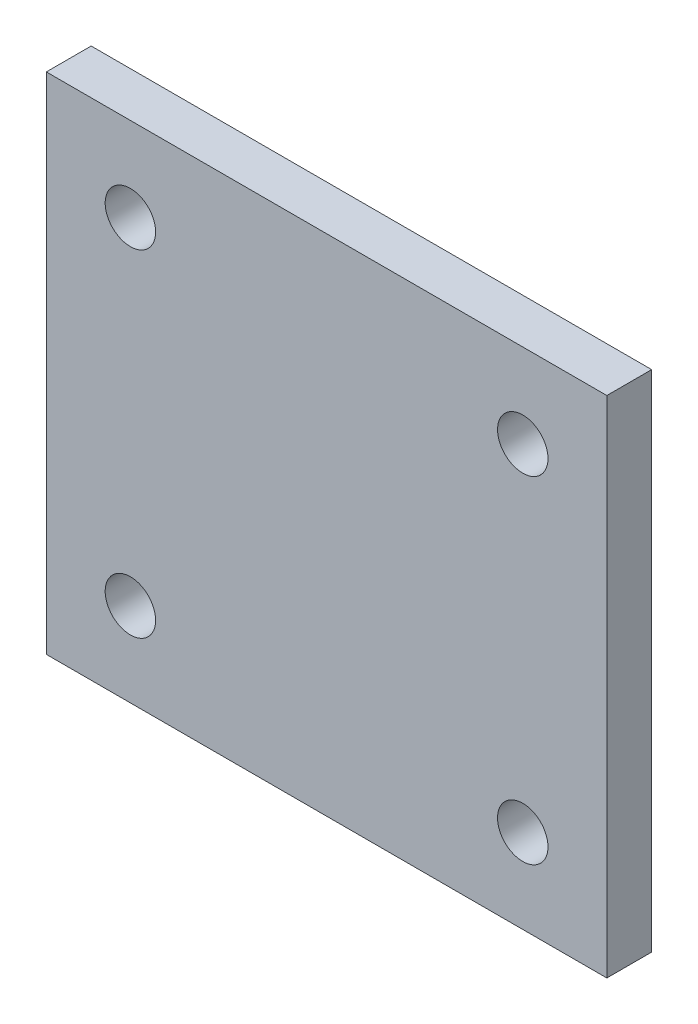
from build123d import *

# Parameters (mm, degrees)
SKETCH_1_W          = 100
SKETCH_1_H          = 90
EXTRUDE_1_DEPTH     = 4
SKETCH_2_R          = 4.5
CUT_EXTRUDE_1_DEPTH = 14


with BuildPart() as part:
    # 草图1 → 凸台-拉伸1 (new, symmetric)
    with BuildSketch(Plane.XY):
        Rectangle(SKETCH_1_W, SKETCH_1_H)
    extrude(amount=EXTRUDE_1_DEPTH, both=True)

    # 草图2 → 切除-拉伸1 (cut, symmetric)
    with BuildSketch(Plane.XY):
        with Locations((-35, -30)):
            Circle(SKETCH_2_R)
        with Locations((35, -30)):
            Circle(SKETCH_2_R)
        with Locations((-35, 30)):
            Circle(SKETCH_2_R)
        with Locations((35, 30)):
            Circle(SKETCH_2_R)
    extrude(amount=CUT_EXTRUDE_1_DEPTH, both=True, mode=Mode.SUBTRACT)


solid = part.part
